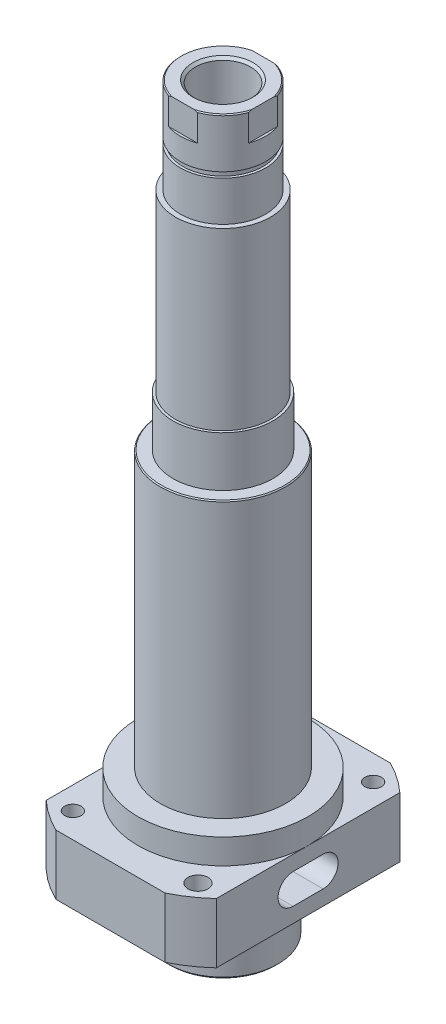
SolidWorks part; units mm, degrees
material "S45C"
ref_plane "Front Plane" through (0, 0, 0) normal (0, 0, 1) x (1, 0, 0)
ref_plane "Top Plane" through (0, 0, 0) normal (0, 1, 0) x (1, 0, 0)
ref_plane "Right Plane" through (0, 0, 0) normal (1, 0, 0) x (0, 0, -1)
sketch "Sketch1" plane through (0, 0, 0) normal (0, 0, 1) x (1, 0, 0)
  line L0 (0, 0) -> (11, 0)
  line L1 (11, 0) -> (11, 12)
  line L2 (11, 12) -> (25, 12)
  line L3 (25, 12) -> (25, 24)
  line L4 (25, 24) -> (17, 24)
  line L5 (0, 148) -> (0, 0)
  line L6 (12.5, 29) -> (12.5, 84)
  line L7 (12.5, 84) -> (10, 84)
  line L8 (10, 84) -> (10, 94)
  line L9 (8.5, 148) -> (0, 148)
  line L10 (17, 24) -> (17, 29)
  line L11 (17, 29) -> (12.5, 29)
  line L12 (10, 94) -> (9.5, 94)
  line L13 (9.5, 94) -> (9.5, 129)
  line L14 (8.5, 148) -> (8.5, 138.1)
  line L15 (8.5, 129) -> (9.5, 129)
  line L16 (8.5, 137) -> (8.5, 129)
  line L17 (8.5, 137) -> (8, 137)
  line L19 (8.5, 138.1) -> (8, 138.1)
  line L20 (8, 137) -> (8, 138.1)
  dimension "D1" = 11
  dimension "D2" = 25
  dimension "D3" = 12
  dimension "D4" = 12
  dimension "D5" = 12.5
  dimension "D6" = 55
  dimension "D7" = 10
  dimension "D8" = 64
  dimension "D9" = 5
  dimension "D10" = 17
  dimension "D11" = 9.5
  dimension "D12" = 10
  dimension "D13" = 8.5
  dimension "D14" = 35
  dimension "D15" = 9.9
  dimension "D16" = 1.1
  dimension "D17" = 8
revolve "Revolve1" add sketch "Sketch1" angle 360 about L5
cosmetic thread "Cosmetic Thread1" parameters "D1"=20, "D2"=20.752
sketch "Sketch7" plane through (0, 24, 0) normal (0, 1, 0) x (1, 0, 0)
  line L1 (17, 22.5) -> (-17, 22.5)
  line L2 (17, 22.5) -> (17, -22.5)
  line L3 (17, -22.5) -> (-17, -22.5)
  line L4 (-17, 22.5) -> (-17, -22.5)
  line L5 (17, 22.5) -> (-17, -22.5) construction
  line L6 (17, -22.5) -> (-17, 22.5) construction
  point P0 (0, 0)
  dimension "D1" = 34
  dimension "D2" = 45
extrude "Cut-Extrude3" cut sketch "Sketch7" against normal blind 25 flip side to cut
hole_wizard "M4 Tapped Hole2" positions "Sketch12" profile "Sketch11" tap size "M4" standard "Gb" end condition through all
sketch "Sketch12" plane through (0, 12, 0) normal (0, -1, 0) x (-1, 0, 0)
  line L1 (-12.5, -17.5) -> (12.5, -17.5) construction
  line L2 (-12.5, -17.5) -> (-12.5, 17.5) construction
  line L3 (-12.5, 17.5) -> (12.5, 17.5) construction
  line L4 (12.5, -17.5) -> (12.5, 17.5) construction
  line L5 (-12.5, -17.5) -> (12.5, 17.5) construction
  line L6 (-12.5, 17.5) -> (12.5, -17.5) construction
  point P0 (-12.5, 17.5)
  point P4 (12.5, -17.5)
  dimension "D1" = 35
  dimension "D2" = 25
sketch "Sketch11" plane through (12.5, 12, -17.5) normal (1, 0, 0) x (0, 0, -1)
  line L0 (0, 0) -> (0, 136)
  line L1 (0, 136) -> (1.65, 136)
  line L2 (1.65, 136) -> (1.65, 0)
  line L5 (1.65, 0) -> (0, 0)
  line L11 (0, -6.35) -> (0, 107.95) construction
  dimension "通孔螺纹孔钻头直径" = 3.3
  dimension "通孔螺纹孔钻头深度" = 136
cosmetic thread "Cosmetic Thread5" parameters "D2"=4
cosmetic thread "Cosmetic Thread7" parameters "D2"=4
sketch "Sketch13" plane through (0, 12, 0) normal (0, -1, 0) x (1, 0, 0)
  line L1 (12.5, 17.5) -> (-12.5, 17.5) construction
  line L2 (12.5, 17.5) -> (12.5, -17.5) construction
  line L3 (12.5, -17.5) -> (-12.5, -17.5) construction
  line L4 (-12.5, 17.5) -> (-12.5, -17.5) construction
  line L5 (12.5, 17.5) -> (-12.5, -17.5) construction
  line L6 (12.5, -17.5) -> (-12.5, 17.5) construction
  circle A0 centre (12.5, 17.5) radius 2
  circle A1 centre (-12.5, -17.5) radius 2
  point P2 (0, 0)
  dimension "D1" = 4
extrude "Cut-Extrude6" cut sketch "Sketch13" against normal blind 25
sketch "Sketch14" plane through (0, 0, 0) normal (0, -1, 0) x (1, 0, 0)
  circle A0 centre (0, 0) radius 5.5
  dimension "D1" = 11
extrude "Cut-Extrude7" cut sketch "Sketch14" against normal through all
chamfer "Chamfer1" distance 0.2 angle 45 2 edges at (0, 84, 12.5) (0, 148, 8.5)
chamfer "Chamfer2" distance 0.5 angle 45 3 edges at (0, 0, 11) (5.5, 148, 0) (5.5, 0, 0)
sketch "Sketch15" plane through (0, 0, 0) normal (0, 0, 1) x (1, 0, 0)
  line L1 (8, 149.7034) -> (12.842, 149.7034)
  line L2 (8, 149.7034) -> (8, 142.5)
  line L3 (8, 142.5) -> (12.842, 142.5)
  line L4 (12.842, 149.7034) -> (12.842, 142.5)
  line L5 (6, 148) -> (-6, 148) construction
  line L6 (8.5, 138.1) -> (8.5, 147.8) construction
  dimension "D1" = 0.5
  dimension "D2" = 5.5
extrude "Cut-Extrude8" cut sketch "Sketch15" against normal mid plane 10
sketch "Sketch16" plane through (-17, 0, 0) normal (-1, 0, 0) x (0, 0, 1)
  line L0 (-3, 18) -> (3, 18) construction
  line L1 (-3, 21) -> (3, 21)
  line L2 (-3, 15) -> (3, 15)
  line L3 (22.5, 18) -> (-22.5, 18) construction
  line L4 (22.5, 24) -> (22.5, 12) construction
  line L5 (-22.5, 12) -> (-22.5, 24) construction
  arc A0 (-3, 21) -> (-3, 15) centre (-3, 18) ccw
  arc A1 (3, 15) -> (3, 21) centre (3, 18) ccw
  point P2 (0, 18)
  dimension "D1" = 3
  dimension "D2" = 6
extrude "Cut-Extrude9" cut sketch "Sketch16" against normal through all
sketch "Sketch17" plane through (0, 0, 0) normal (1, 0, 0) x (0, 0, -1)
  line L0 (2.8723, 142.5) -> (-2.8723, 142.5) construction
  line L1 (11.089, 150.5485) -> (8, 150.5485)
  line L2 (11.089, 150.5485) -> (11.089, 142.5)
  line L3 (11.089, 142.5) -> (8, 142.5)
  line L4 (8, 150.5485) -> (8, 142.5)
  line L5 (-10.9985, 151.4673) -> (-8, 151.4673)
  line L6 (-10.9985, 151.4673) -> (-10.9985, 142.5)
  line L7 (-10.9985, 142.5) -> (-8, 142.5)
  line L8 (-8, 151.4673) -> (-8, 142.5)
  line L9 (8.5, 138.1) -> (8.5, 147.8) construction
  line L10 (0, 0) -> (0, 168.6056) construction
  dimension "D1" = 0.5
extrude "Cut-Extrude10" cut sketch "Sketch17" against normal mid plane 10
